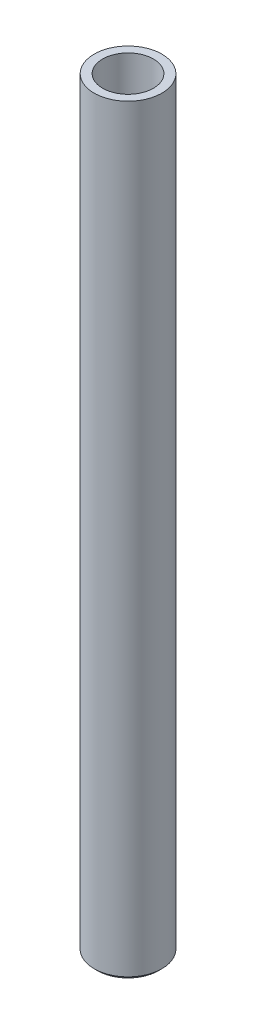
SolidWorks part; units mm, degrees
material "普通碳钢"
ref_plane "Front Plane" through (0, 0, 0) normal (0, 0, 1) x (1, 0, 0)
ref_plane "Top Plane" through (0, 0, 0) normal (0, 1, 0) x (1, 0, 0)
ref_plane "Right Plane" through (0, 0, 0) normal (1, 0, 0) x (0, 0, -1)
sketch "Sketch1" plane through (0, 0, 0) normal (0, 1, 0) x (1, 0, 0)
  circle A0 centre (0, 0) radius 2
  dimension "D1" = 4
extrude "Boss-Extrude1" add sketch "Sketch1" along normal blind 45
chamfer "Chamfer1" distance 0.2 angle 45 1 edges at (0, 0, 2)
sketch "Sketch3" plane through (0, 45, 0) normal (0, 1, 0) x (1, 0, 0)
  circle A0 centre (0, 0) radius 1.5
  dimension "D1" = 3
extrude "Cut-Extrude1" cut sketch "Sketch3" against normal blind 3
